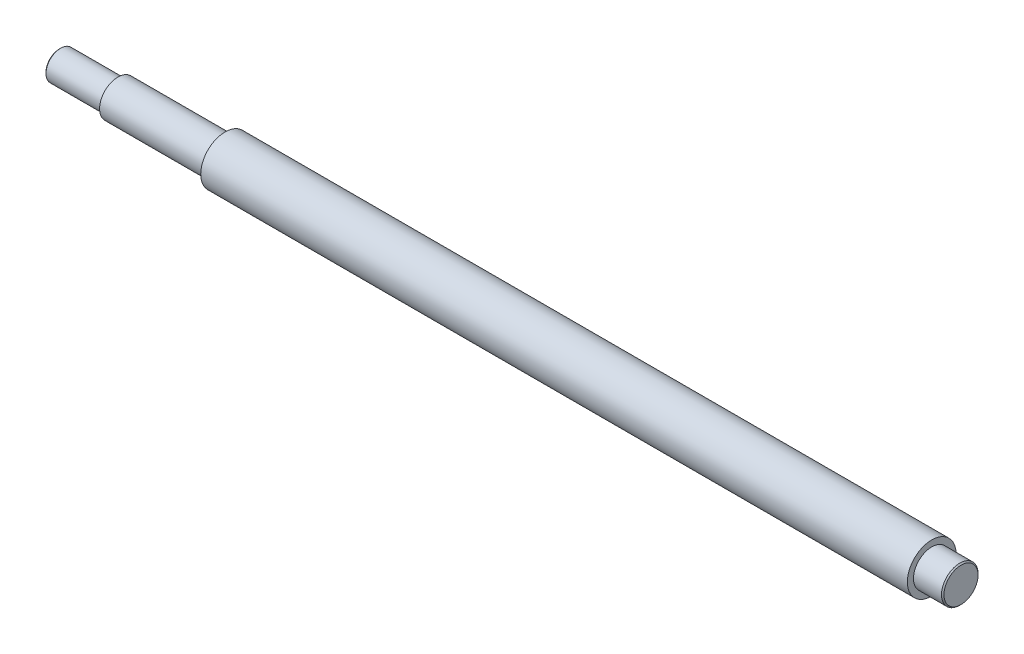
SolidWorks part; units mm, degrees
material "标准件"
ref_plane "前视基准面" through (0, 0, 0) normal (0, 0, 1) x (1, 0, 0)
ref_plane "上视基准面" through (0, 0, 0) normal (0, 1, 0) x (1, 0, 0)
ref_plane "右视基准面" through (0, 0, 0) normal (1, 0, 0) x (0, 0, -1)
sketch "草图1" plane through (0, 0, 0) normal (0, 1, 0) x (1, 0, 0)
  line L0 (0, 0) -> (370, 0) construction
  line L1 (0, 0) -> (0, 6)
  line L2 (0, 6) -> (24, 6)
  line L3 (24, 6) -> (24, 7.5)
  line L4 (24, 7.5) -> (68, 7.5)
  line L5 (68, 7.5) -> (68, 10)
  line L6 (68, 10) -> (358, 10)
  line L7 (358, 10) -> (358, 7.5)
  line L8 (358, 7.5) -> (370, 7.5)
  line L9 (370, 7.5) -> (370, 0)
  line L10 (0, 0) -> (370, 0)
  dimension "D1" = 44
  dimension "D2" = 15
  dimension "D3" = 12
  dimension "D4" = 20
  dimension "D5" = 24
  dimension "D6" = 12
  dimension "D7" = 15
  dimension "D8" = 370
revolve "旋转1" add sketch "草图1" angle 360 about L0
cosmetic thread "装饰螺纹线1" parameters "D2"=17.294
cosmetic thread "装饰螺纹线2" parameters "D1"=10, "D2"=11.797
ref_plane "基准面1" through (0, -6, 0) normal (0, -1, 0) x (-1, 0, 0)
sketch "草图2" plane through (0, -6, 0) normal (0, -1, 0) x (-1, 0, 0)
  line L0 (-24, 0) -> (0, 0) construction
  line L1 (-24, -7.5) -> (-24, 7.5) construction
  line L2 (-21, 0) -> (-3, 0) construction
  line L3 (-21, 2) -> (-3, 2)
  line L4 (-21, -2) -> (-3, -2)
  line L5 (0, -6) -> (0, 6) construction
  arc A0 (-21, 2) -> (-21, -2) centre (-21, 0) ccw
  arc A1 (-3, -2) -> (-3, 2) centre (-3, 0) ccw
  point P7 (-12, 0)
  dimension "D1" = 4
  dimension "D2" = 1
extrude "切除-拉伸1" cut sketch "草图2" against normal blind 2.2
chamfer "倒角1" distance 0.5 angle 45 2 edges at (370, 0, 7.5) (0, 0, 6)
